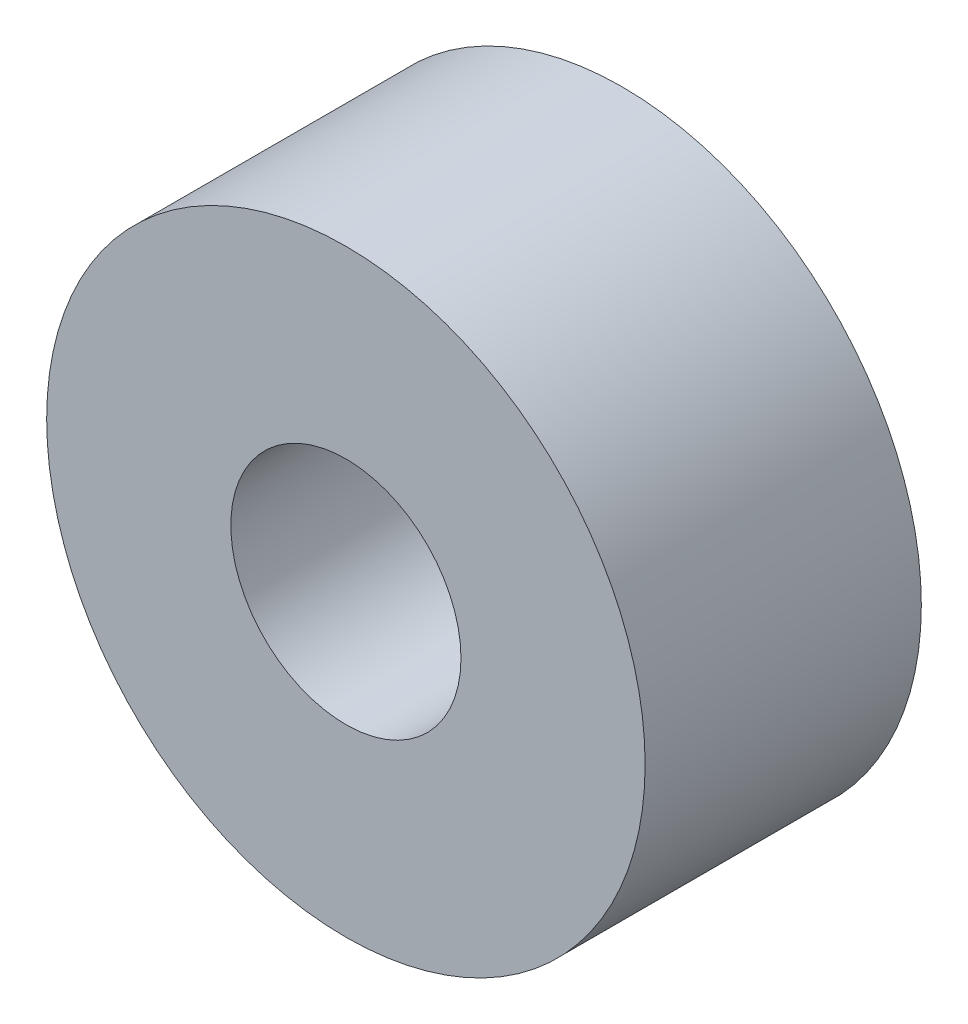
from build123d import *

# Parameters (mm, degrees)
SKETCH1_R           = 6.5
SKETCH1_R_2         = 2.5
BOSS_EXTRUDE1_DEPTH = 6


with BuildPart() as part:
    # Sketch1 → Boss-Extrude1 (new body)
    with BuildSketch(Plane.XY.offset(-6)):
        Circle(SKETCH1_R)
        Circle(SKETCH1_R_2, mode=Mode.SUBTRACT)
    extrude(amount=BOSS_EXTRUDE1_DEPTH)


solid = part.part
